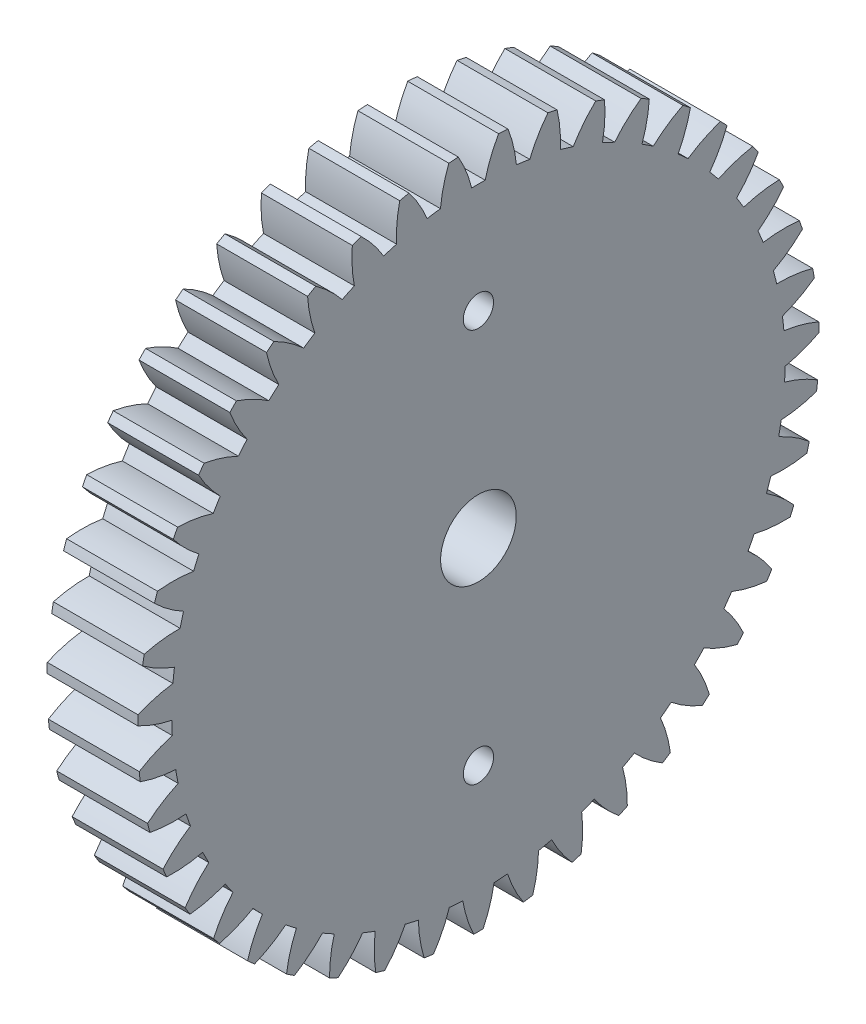
SolidWorks part; units mm, degrees
ref_plane "Plane1" through (0, 0, 0) normal (0, 0, 1) x (1, 0, 0)
ref_plane "Plane2" through (0, 0, 0) normal (0, 1, 0) x (1, 0, 0)
ref_plane "Plane3" through (0, 0, 0) normal (1, 0, 0) x (0, 0, -1)
sketch "HoldingSke" plane through (0, 0, 0) normal (0, 1, 0) x (1, 0, 0)
  line L0 (0, 0) -> (0.7314, -0.682)
  line L1 (-15, 0) -> (100, 0) construction
  line L2 (0, 0) -> (-2.1039, 2.3779)
  line L3 (0, 0) -> (-11.863, 4.5341)
  line L4 (0, 0) -> (6.316, 5.8897)
  line L5 (0, 0) -> (-46.8476, -17.4728)
  line L6 (0, 0) -> (-4.9738, -3.3558)
  line L7 (-2.1039, 2.3779) -> (8.6586, 51.2059)
  line L8 (-76.2, 54.61) -> (-75.3, 54.61)
  line L9 (-71.009, 38.7566) -> (-53.1078, 45.2721)
  line L10 (-76.2, 71.12) -> (104.1128, 71.12)
  line L11 (0, 0) -> (-6, 0)
  line L12 (-76.2, 101.6) -> (-76.162, 101.6)
  line L13 (24.9733, 27.94) -> (52.9518, 28.4284)
  line L14 (24.9733, 27.94) -> (24.9743, 27.94)
  line L15 (24.9733, 27.94) -> (100.4006, 29.5858)
  line L16 (-63.627, -1) -> (-12.827, -1)
  circle A0 centre (0, 0) radius 2.5
  circle A1 centre (0, 0) radius 20.249
  circle A2 centre (0, 0) radius 37.5
  circle A3 centre (0, 0) radius 2.5
sketch "BasProSke" plane through (0, 0, 0) normal (0, 1, 0) x (1, 0, 0)
  line L0 (-10, 0) -> (60, 0) construction
  line L1 (0, 0) -> (0, 22.5)
  line L2 (0, 0) -> (6, 0)
  line L3 (6, 0) -> (6, 22.5)
  line L4 (6, 22.5) -> (0, 22.5)
revolve "Base-Revolve" add sketch "BasProSke" angle 360 about L0
sketch "TooCutSke" plane through (0, 0, 0) normal (1, 0, 0) x (0, 0, -1)
  line L1 (0, 0) -> (0, 107) construction
  line L2 (0, 0) -> (-0.8517, 21.4831) construction
  line L3 (0, 0) -> (-3.137, 42.8613) construction
  line L4 (-0.8517, 21.4831) -> (-1.5685, 21.4307) construction
  arc A0 (0.4449, 20.2441) -> (-0.4449, 20.2441) centre (0, 0) ccw
  arc A1 (1.3459, 22.4852) -> (-1.3459, 22.4852) centre (0, 0) ccw
  circle A2 centre (0, 0) radius 21.5 construction
  circle A3 centre (0, 0) radius 20.2034 construction
  arc A4 (-0.4449, 20.2441) -> (-1.3459, 22.4852) centre (-8.7955, 18.1883) ccw
  arc A5 (1.3459, 22.4852) -> (0.4449, 20.2441) centre (8.7955, 18.1883) ccw
extrude "ToothCut" cut sketch "TooCutSke" along normal through all
fillet "Breaks" [suppressed] radius 0.02
fillet "RootFillets" [suppressed] radius 0.251
pattern_circular "TeethCuts" count 43 every 8.372 about axis through (-10, 0, 0) along (1, 0, 0) of "ToothCut", "RootFillets", "Breaks"
sketch "HubNeaOneSke" plane through (0, 0, 0) normal (-1, 0, 0) x (0, 0, 1)
  circle A0 centre (0, 0) radius 20.249
extrude "HubNearOne" [suppressed] add sketch "HubNeaOneSke" along normal blind 44.0001
sketch "HubNeaBotSke" plane through (0, 0, 0) normal (-1, 0, 0) x (0, 0, 1)
  circle A0 centre (0, 0) radius 20.249
extrude "HubNearBoth" [suppressed] add sketch "HubNeaBotSke" along normal blind 22
ref_plane "FarPln" through (6, 0, 0) normal (1, 0, 0) x (0, 0, -1)
sketch "HubFarSke" plane through (6, 0, 0) normal (1, 0, 0) x (0, 0, -1)
  circle A0 centre (0, 0) radius 20.249
extrude "HubFar" [suppressed] add sketch "HubFarSke" along normal blind 22
sketch "BorSke" plane through (0, 0, 0) normal (1, 0, 0) x (0, 0, -1)
  circle A0 centre (0, 0) radius 2.5
extrude "Bore" cut sketch "BorSke" along normal mid plane 100.0001
sketch "KeySke" plane through (0, 0, 0) normal (1, 0, 0) x (0, 0, -1)
  line L0 (-1, 0) -> (-1, 3.4)
  line L1 (-1, 3.4) -> (1, 3.4)
  line L2 (1, 3.4) -> (1, 0)
  line L3 (0, 0) -> (0, 34) construction
  line L4 (-1, 0) -> (1, 0)
extrude "Keyway" [suppressed] cut sketch "KeySke" along normal mid plane 100.0001
pattern_circular "Keyway2" [suppressed] count 2 every 90 about axis through (-10, 0, 0) along (1, 0, 0)
sketch "Sketch1" plane through (6, 0, 0) normal (1, 0, 0) x (0, 0, -1)
  circle A0 centre (0, 13) radius 1
  circle A1 centre (0, -13) radius 1
  circle A2 centre (0, 0) radius 2.5 construction
  dimension "D1" = 2
  dimension "D2" = 2
  dimension "D3" = 26
  dimension "D4" = 13
extrude "Cut-Extrude1" cut sketch "Sketch1" against normal through all
equation "' \"Module@HoldingSke\" = 6.35"
equation "' \"Num_teeth@HoldingSke\" = 12"
equation "' \"Ap@HoldingSke\" =  20"
equation "' \"Ap@HoldingSke\" = 20"
equation "' \"Width@HoldingSke\" = 0.5 * 25.4"
equation "' \"Hub_dia@HoldingSke\"= 1 * 25.4"
equation "' \"Hub_dia@HoldingSke\" = 1 * 25.4"
equation "' \"Overall_len@HoldingSke\" = 1.0 * 25.4"
equation "' \"Bore@HoldingSke\" = 0.75 * 25.4"
equation "' \"T_dim@HoldingSke\" = 0.1 * 25.4"
equation "' \"Width@KeySke\" = 0.25 * 25.4"
equation "' \"Show_teeth@HoldingSke\" = 13"
equation "' \"Backlash@HoldingSke\" = 0.009 * 25.4"
equation "' \"Addendum_fac@HoldingSke\" = 1.0"
equation "' \"Dedendum_fac@HoldingSke\" = 1.25"
equation "' \"Dedendum_add@HoldingSke\" = 0.00005 * 25.4"
equation "' \"Clearance_fac@HoldingSke\" = 0.25"
equation "\"Pitch@HoldingSke\" = 1 / \"Module@HoldingSke\""
equation "\"Overcut_dia@TooCutSke\" = (\"Num_teeth@HoldingSke\" + 2 * \"Addendum_fac@HoldingSke\") / \"Pitch@HoldingSke\" + 0.002 * 25.4"
equation "\"Pitch_dia@TooCutSke\" = \"Num_teeth@HoldingSke\" / \"Pitch@HoldingSke\""
equation "\"Base_dia@TooCutSke\" = \"Num_teeth@HoldingSke\" / \"Pitch@HoldingSke\" * cos((\"Ap@HoldingSke\"  * 3.14159265 / 180))"
equation "\"Root_dia@TooCutSke\" = (\"Num_teeth@HoldingSke\" + 2) / \"Pitch@HoldingSke\" - 2 * (\"Addendum_fac@HoldingSke\" + \"Dedendum_fac@HoldingSke\") / \"Pitch@HoldingSke\" - \"Dedendum_add@HoldingSke\" * 2"
equation "\"Half_ang@TooCutSke\" = 180 / \"Num_teeth@HoldingSke\""
equation "\"Half_CT@TooCutSke\" = \"Num_teeth@HoldingSke\" / \"Pitch@HoldingSke\" * sin((3.14159265 / 2 / \"Num_teeth@HoldingSke\")) / 2 - 7 * \"Backlash@HoldingSke\" / 4"
equation "\"Flank_rad@TooCutSke\" = \"Num_teeth@HoldingSke\" / \"Pitch@HoldingSke\" / 5"
equation "\"Radius@RootFillets\" = \"Clearance_fac@HoldingSke\" / \"Pitch@HoldingSke\" + \"Dedendum_add@HoldingSke\""
equation "\"Break_rad@Breaks\" = 0.02 / \"Pitch@HoldingSke\""
equation "\"Thickness@HoldingSke\" = \"Width@HoldingSke\""
equation "\"OAL@HoldingSke\" = \"Thickness@HoldingSke\""
equation "\"MHD@HoldingSke\" = (\"Num_teeth@HoldingSke\" + 2) / \"Pitch@HoldingSke\" - 2 * (\"Addendum_fac@HoldingSke\" + \"Dedendum_fac@HoldingSke\")  / \"Pitch@HoldingSke\" - \"Dedendum_add@HoldingSke\" * 2"
equation "\"MBD@HoldingSke\" = (\"Num_teeth@HoldingSke\" + 2) / \"Pitch@HoldingSke\" - 2 * (\"Addendum_fac@HoldingSke\" + \"Dedendum_fac@HoldingSke\")  / \"Pitch@HoldingSke\" - \"Dedendum_add@HoldingSke\" * 2 - 0.002 * 25.4"
equation "\"MHD@HoldingSke\" = ((sgn( \"MHD@HoldingSke\" - \"Hub_dia@HoldingSke\" )-1)*( \"MHD@HoldingSke\" - \"Hub_dia@HoldingSke\" ))/-2+ \"Hub_dia@HoldingSke\""
equation "\"MBD@HoldingSke\" = ((sgn( \"MBD@HoldingSke\" - \"Bore@HoldingSke\" )-1)*( \"MBD@HoldingSke\" - \"Bore@HoldingSke\" ))/-2+ \"Bore@HoldingSke\""
equation "\"OAL@HoldingSke\" = ((sgn( \"OAL@HoldingSke\" - \"Overall_len@HoldingSke\" )+1)*( \"OAL@HoldingSke\" - \"Overall_len@HoldingSke\" ))/2 + \"Overall_len@HoldingSke\" + 0.000002 * 25.4"
equation "\"Num_teeth@TeethCuts\" = int( \"Show_teeth@HoldingSke\" ) + 1"
equation "\"Num_teeth@TeethCuts\" = ((sgn( \"Num_teeth@TeethCuts\" - \"Num_teeth@HoldingSke\" )-1)*( \"Num_teeth@TeethCuts\" - \"Num_teeth@HoldingSke\" ))/-2+ \"Num_teeth@HoldingSke\""
equation "\"Num_teeth@TeethCuts\" = ((sgn( \"Num_teeth@TeethCuts\" - 2.0)+1)*( \"Num_teeth@TeethCuts\" - 2.0))/2 +2.0"
equation "\"Angle@TeethCuts\" = 360.0 / \"Num_teeth@HoldingSke\""
equation "\"Diameter@BasProSke\" = (\"Num_teeth@HoldingSke\" + 2 * \"Addendum_fac@HoldingSke\") / \"Pitch@HoldingSke\""
equation "\"Thickness@BasProSke\"  = \"Thickness@HoldingSke\""
equation "' \"Fillet_rad@BasProSke\" =  \"Thickness@HoldingSke\" * 0.05"
equation "' \"Fillet_rad@BasProSke\" = \"Thickness@HoldingSke\" * 0.05"
equation "\"MHD@HoldingSke\" = ((sgn( \"MHD@HoldingSke\" - \"Root_dia@TooCutSke\" )-1)*( \"MHD@HoldingSke\" - \"Root_dia@TooCutSke\" ))/-2+ \"Root_dia@TooCutSke\""
equation "\"Diameter@HubNeaOneSke\" = \"MHD@HoldingSke\""
equation "\"Length@HubNearOne\" = \"OAL@HoldingSke\" - \"Thickness@BasProSke\""
equation "\"Diameter@HubNeaBotSke\" = \"MHD@HoldingSke\""
equation "\"Length@HubNearBoth\" = ( \"OAL@HoldingSke\" - \"Thickness@BasProSke\" ) / 2.0"
equation "\"Thickness@FarPln\" = \"Thickness@BasProSke\""
equation "\"Diameter@HubFarSke\" = \"MHD@HoldingSke\""
equation "\"Length@HubFar\" = ( \"OAL@HoldingSke\" - \"Thickness@BasProSke\" ) / 2.0"
equation "\"Diameter@BorSke\" = \"MBD@HoldingSke\""
equation "\"D1@Bore\" = \"OAL@HoldingSke\" * 2.0"
equation "\"D1@Keyway\" = \"OAL@HoldingSke\" * 2.0"
equation "\"Offset@KeySke\" = \"T_dim@HoldingSke\" + \"MBD@HoldingSke\" / 2.0"
